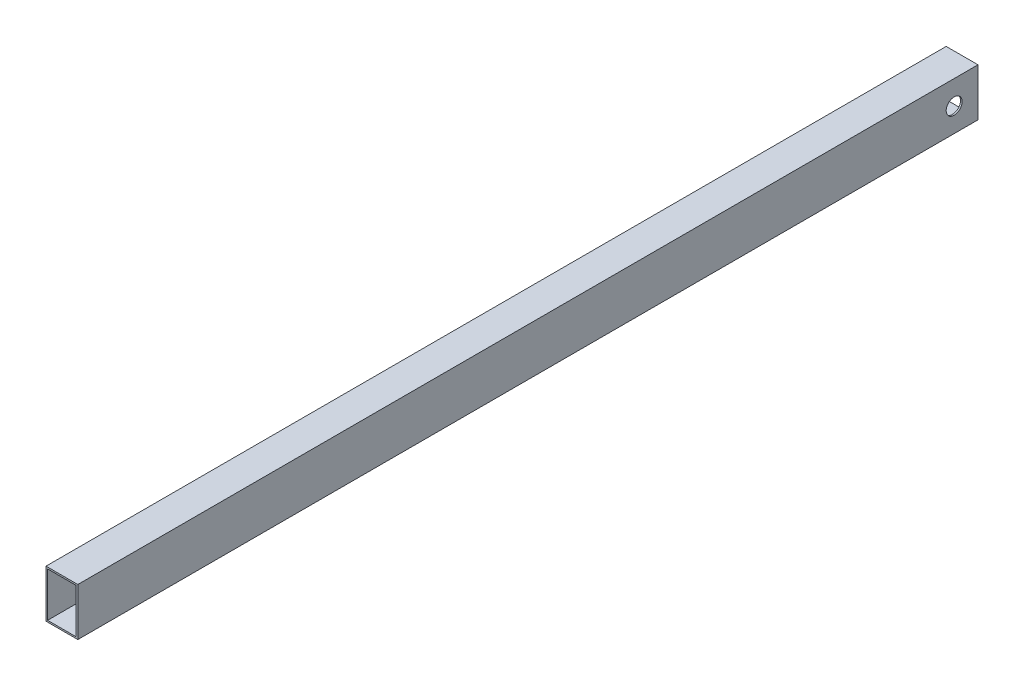
SolidWorks part; units mm, degrees
ref_plane "Front Plane" through (0, 0, 0) normal (0, 0, 1) x (1, 0, 0)
ref_plane "Top Plane" through (0, 0, 0) normal (0, 1, 0) x (1, 0, 0)
ref_plane "Right Plane" through (0, 0, 0) normal (1, 0, 0) x (0, 0, -1)
sketch "Sketch1" plane through (0, 0, 0) normal (0, 0, 1) x (1, 0, 0)
  line L1 (0, 0) -> (20, 0)
  line L2 (0, 0) -> (0, -30)
  line L3 (0, -30) -> (20, -30)
  line L4 (20, 0) -> (20, -30)
  line L8 (1, -1) -> (19, -1)
  line L9 (19, -1) -> (19, -29)
  line L10 (1, -29) -> (19, -29)
  line L11 (1, -1) -> (1, -29)
  dimension "D1" = 20
  dimension "D2" = 30
  dimension "D3" = 1
extrude "Boss-Extrude1" add sketch "Sketch1" along normal blind 566
sketch "Sketch3" plane through (0, 0, 0) normal (-1, 0, 0) x (0, 0, 1)
  line L0 (536, -30) -> (566, -30)
  line L2 (596, -27) -> (596, -3)
  line L3 (593, 0) -> (566, 0)
  line L4 (566, 0) -> (536, 0)
  line L5 (566, 0) -> (0, 0) construction
  line L6 (566, -30) -> (0, -30) construction
  line L7 (566, -30) -> (593, -30)
  line L8 (536, -30) -> (536, 0)
  arc A0 (596, -27) -> (593, -30) centre (593, -27) cw
  arc A1 (596, -3) -> (593, 0) centre (593, -3) ccw
  point P14 (596, -30)
  dimension "D3" = 3
  dimension "D4" = 3
  dimension "D1" = 30
  dimension "D2" = 30
ref_plane "Plane4" through (10, 0, 0) normal (1, 0, 0) x (0, 0, -1)
sketch "Sketch4" plane through (0, 0, 0) normal (-1, 0, 0) x (0, 0, 1)
  line L0 (0, -15) -> (566, -15) construction
  line L1 (0, 0) -> (0, -30) construction
  line L2 (566, 0) -> (566, -30) construction
  circle A0 centre (15, -15) radius 5
  dimension "D1" = 10
  dimension "D2" = 15
extrude "Cut-Extrude1" cut sketch "Sketch4" against normal through all
